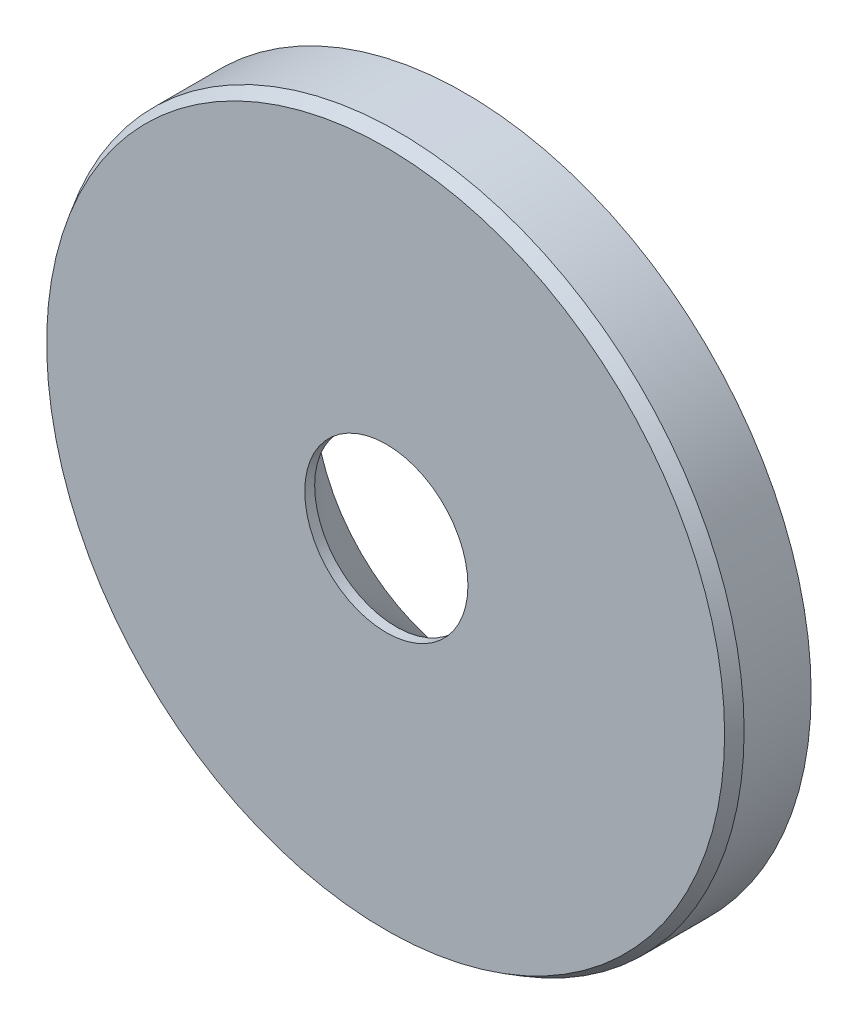
from build123d import *
from OCP.BRepFilletAPI import BRepFilletAPI_MakeChamfer

# Parameters (mm, degrees)
SKETCH1_R                                            = 14
BOSS_EXTRUDE1_DEPTH                                  = 3.5
CHAMFER1_SIZE                                        = 0.5
CHAMFER1_SIZE2                                       = 0.288675135
CSK_FOR_M6_HEXAGON_LOBULAR_SOCKET_RAISED_D           = 6.6
CSK_FOR_M6_HEXAGON_LOBULAR_SOCKET_RAISED_DEPTH       = 6.5
CSK_FOR_M6_HEXAGON_LOBULAR_SOCKET_RAISED_CSINK_D     = 12.8
CSK_FOR_M6_HEXAGON_LOBULAR_SOCKET_RAISED_CSINK_ANGLE = 90
CSK_FOR_M6_HEXAGON_LOBULAR_SOCKET_RAISED_TIP         = 1.982840043


with BuildPart() as part:
    # Sketch1 → Boss-Extrude1 (new body)
    with BuildSketch(Plane.XY):
        Circle(SKETCH1_R)
    extrude(amount=BOSS_EXTRUDE1_DEPTH)

    # Chamfer1: one chamfer whose edges measure the first distance from different faces: ONE call of the kernel's chamfer builder (chamfer() names one face for all edges)
    chamfer1_edges_1 = [part.edges().sort_by_distance(p)[0] for p in [
        (-14, 0, 0),
    ]]
    chamfer1_side_1 = [part.faces().sort_by_distance(p)[0] for p in [
        (0, 0, 0),
    ]]
    chamfer1_edges_2 = [part.edges().sort_by_distance(p)[0] for p in [
        (-14, 0, 3.5),
    ]]
    chamfer1_side_2 = [part.faces().sort_by_distance(p)[0] for p in [
        (-14, 0, 1.75),
    ]]
    chamfer1 = BRepFilletAPI_MakeChamfer(part.part.solid().wrapped)
    for e in chamfer1_edges_1:
        chamfer1.Add(CHAMFER1_SIZE, CHAMFER1_SIZE2, e.wrapped, chamfer1_side_1[0].wrapped)  # the first distance lies on this face
    for e in chamfer1_edges_2:
        chamfer1.Add(CHAMFER1_SIZE, CHAMFER1_SIZE2, e.wrapped, chamfer1_side_2[0].wrapped)  # the first distance lies on this face
    add(Compound.cast(chamfer1.Shape()), mode=Mode.REPLACE)

    # CSK for M6 Hexagon lobular socket raised CTSK head screws1
    with Locations(Plane(origin=(0.028531749, 0.017266162, 0), x_dir=(-1, 0, 0), z_dir=(0, 0, -1))):
        with Locations((0, 0)):
            CounterSinkHole(CSK_FOR_M6_HEXAGON_LOBULAR_SOCKET_RAISED_D / 2, CSK_FOR_M6_HEXAGON_LOBULAR_SOCKET_RAISED_CSINK_D / 2, depth=CSK_FOR_M6_HEXAGON_LOBULAR_SOCKET_RAISED_DEPTH, counter_sink_angle=CSK_FOR_M6_HEXAGON_LOBULAR_SOCKET_RAISED_CSINK_ANGLE)
            with Locations((0, 0, -(CSK_FOR_M6_HEXAGON_LOBULAR_SOCKET_RAISED_DEPTH + CSK_FOR_M6_HEXAGON_LOBULAR_SOCKET_RAISED_TIP / 2))):  # 118° drill point
                Cone(0, CSK_FOR_M6_HEXAGON_LOBULAR_SOCKET_RAISED_D / 2, CSK_FOR_M6_HEXAGON_LOBULAR_SOCKET_RAISED_TIP, mode=Mode.SUBTRACT)


solid = part.part
